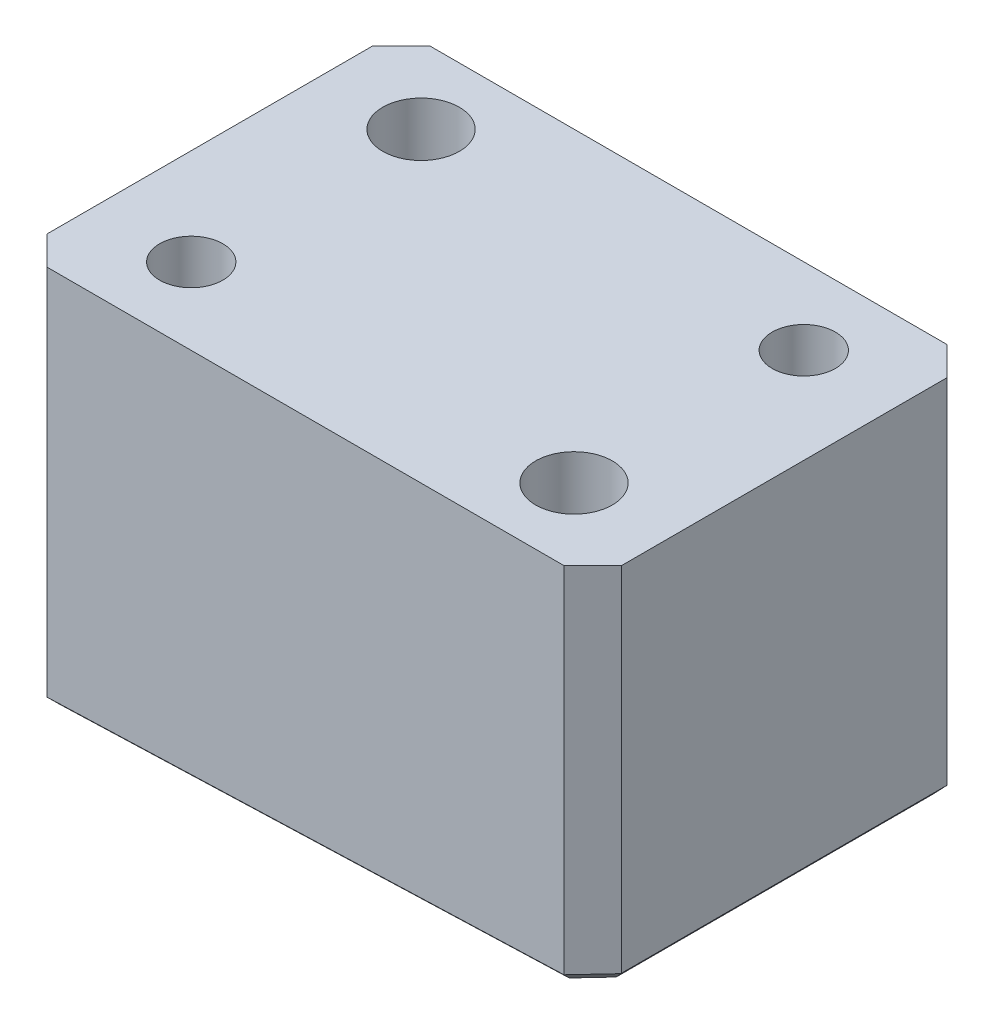
SolidWorks part; units mm, degrees
ref_plane "Front Plane" through (0, 0, 0) normal (0, 0, 1) x (1, 0, 0)
ref_plane "Top Plane" through (0, 0, 0) normal (0, 1, 0) x (1, 0, 0)
ref_plane "Right Plane" through (0, 0, 0) normal (1, 0, 0) x (0, 0, -1)
sketch "Sketch2" plane through (0, 0, 0) normal (0, 0, 1) x (1, 0, 0)
  line L0 (-37.5815, 20.6301) -> (22.4185, 22.7253)
  line L1 (-37.5815, 60.6301) -> (22.4185, 60.6301)
  line L2 (-37.5815, 60.6301) -> (-37.5815, 20.6301)
  line L5 (22.4185, 60.6301) -> (22.4185, 22.7253)
  dimension "D1" = 60
  dimension "D2" = 40
  dimension "D3" = 2
extrude "Boss-Extrude1" add sketch "Sketch2" along normal blind 40
chamfer "Chamfer1" distance 3 angle 45 4 edges at (-37.5815, 40.6301, 0) (22.4185, 41.6777, 0) (22.4185, 41.6777, 40) (-37.5815, 40.6301, 40)
chamfer "Chamfer2" distance 1 angle 45 8 edges at (20.9185, 22.6729, 38.5) (22.4185, 22.7253, 20) (20.9185, 22.6729, 1.5) (-7.5815, 21.6777, 0) (-36.0815, 20.6824, 1.5) (-37.5815, 20.6301, 20) (-36.0815, 20.6824, 38.5) (-7.5815, 21.6777, 40)
sketch "Sketch3" plane through (-0.7653, 21.9157, 0) normal (0.0349, -0.9994, 0) x (0.9994, 0.0349, 0)
  line L0 (23.2342, 37) -> (23.2342, 3) construction
  line L1 (-26.7658, 32) -> (13.2342, 32)
  line L2 (-26.7658, 32) -> (-26.7658, 8)
  line L3 (-26.7658, 8) -> (13.2342, 8)
  line L4 (13.2342, 32) -> (13.2342, 8)
  line L5 (-33.8018, 40) -> (20.2311, 40) construction
  dimension "D1" = 24
  dimension "D2" = 40
  dimension "D3" = 10
  dimension "D4" = 8
sketch "Sketch7" plane through (0, 60.6301, 0) normal (0, 1, 0) x (1, 0, 0)
  line L4 (-27.5148, -32) -> (12.4608, -32)
  line L5 (12.4608, -32) -> (12.4608, -8)
  line L6 (12.4608, -8) -> (-27.5148, -8)
  line L7 (-27.5148, -8) -> (-27.5148, -32)
  line L8 (-27.5148, -32) -> (12.4608, -32)
  line L9 (12.4608, -32) -> (12.4608, -8)
  line L10 (12.4608, -8) -> (-27.5148, -8)
  line L11 (-27.5148, -8) -> (-27.5148, -32)
  dimension "D1" = 0
hole_wizard "Hole2" positions "Sketch8" profile "Sketch9" legacy
sketch "Sketch8" plane through (0, 60.6301, 0) normal (0, 1, 0) x (1, 0, 0)
  point P8 (-27.5148, -32)
  point P11 (12.4608, -8)
sketch "Sketch9" plane through (-27.5148, 60.6301, 32) normal (1, 0, 0) x (0, 0, 1)
  line L0 (0, 0) -> (0, 20)
  line L1 (0, 20) -> (3.3, 20)
  line L2 (3.3, 20) -> (3.3, 0)
  line L3 (3.3, 0) -> (0, 0)
  line L4 (0, 110) -> (0, -10) construction
  dimension "直径" = 6.6
  dimension "深度" = 20
hole_wizard "Hole3" positions "Sketch10" profile "Sketch11" legacy
sketch "Sketch10" plane through (0, 40.6301, 0) normal (0, 1, 0) x (1, 0, 0)
  point P9 (-27.5148, -32)
  point P12 (12.4608, -8)
sketch "Sketch11" plane through (-27.5148, 40.6301, 32) normal (1, 0, 0) x (0, 0, 1)
  line L0 (0, 0) -> (0, 19.9663)
  line L1 (0, 19.9663) -> (5.5, 19.9663)
  line L2 (5.5, 19.9663) -> (5.5, 0)
  line L3 (5.5, 0) -> (0, 0)
  line L4 (0, 110) -> (0, -10) construction
  dimension "直径" = 11
  dimension "深度" = 19.9663
hole_wizard "Size mm blind hole 1" positions "Sketch12" profile "Sketch13" hole size "Ø8.0" standard "GB"
sketch "Sketch12" plane through (0, 60.6301, 0) normal (0, 1, 0) x (1, 0, 0)
  point P8 (-27.5148, -8)
  point P11 (12.4608, -32)
sketch "Sketch13" plane through (-27.5148, 60.6301, 8) normal (1, 0, 0) x (0, 0, 1)
  line L0 (0, 0) -> (0, 14.9034)
  line L1 (0, 14.9034) -> (4, 12.5)
  line L2 (4, 12.5) -> (4, 0)
  line L5 (4, 0) -> (0, 0)
  line L10 (0, 14.9034) -> (-4, 12.5) construction
  line L11 (0, -6.35) -> (0, 107.95) construction
  dimension "孔直径" = 8
  dimension "孔深度" = 12.5
  dimension "导头角度" = 118
